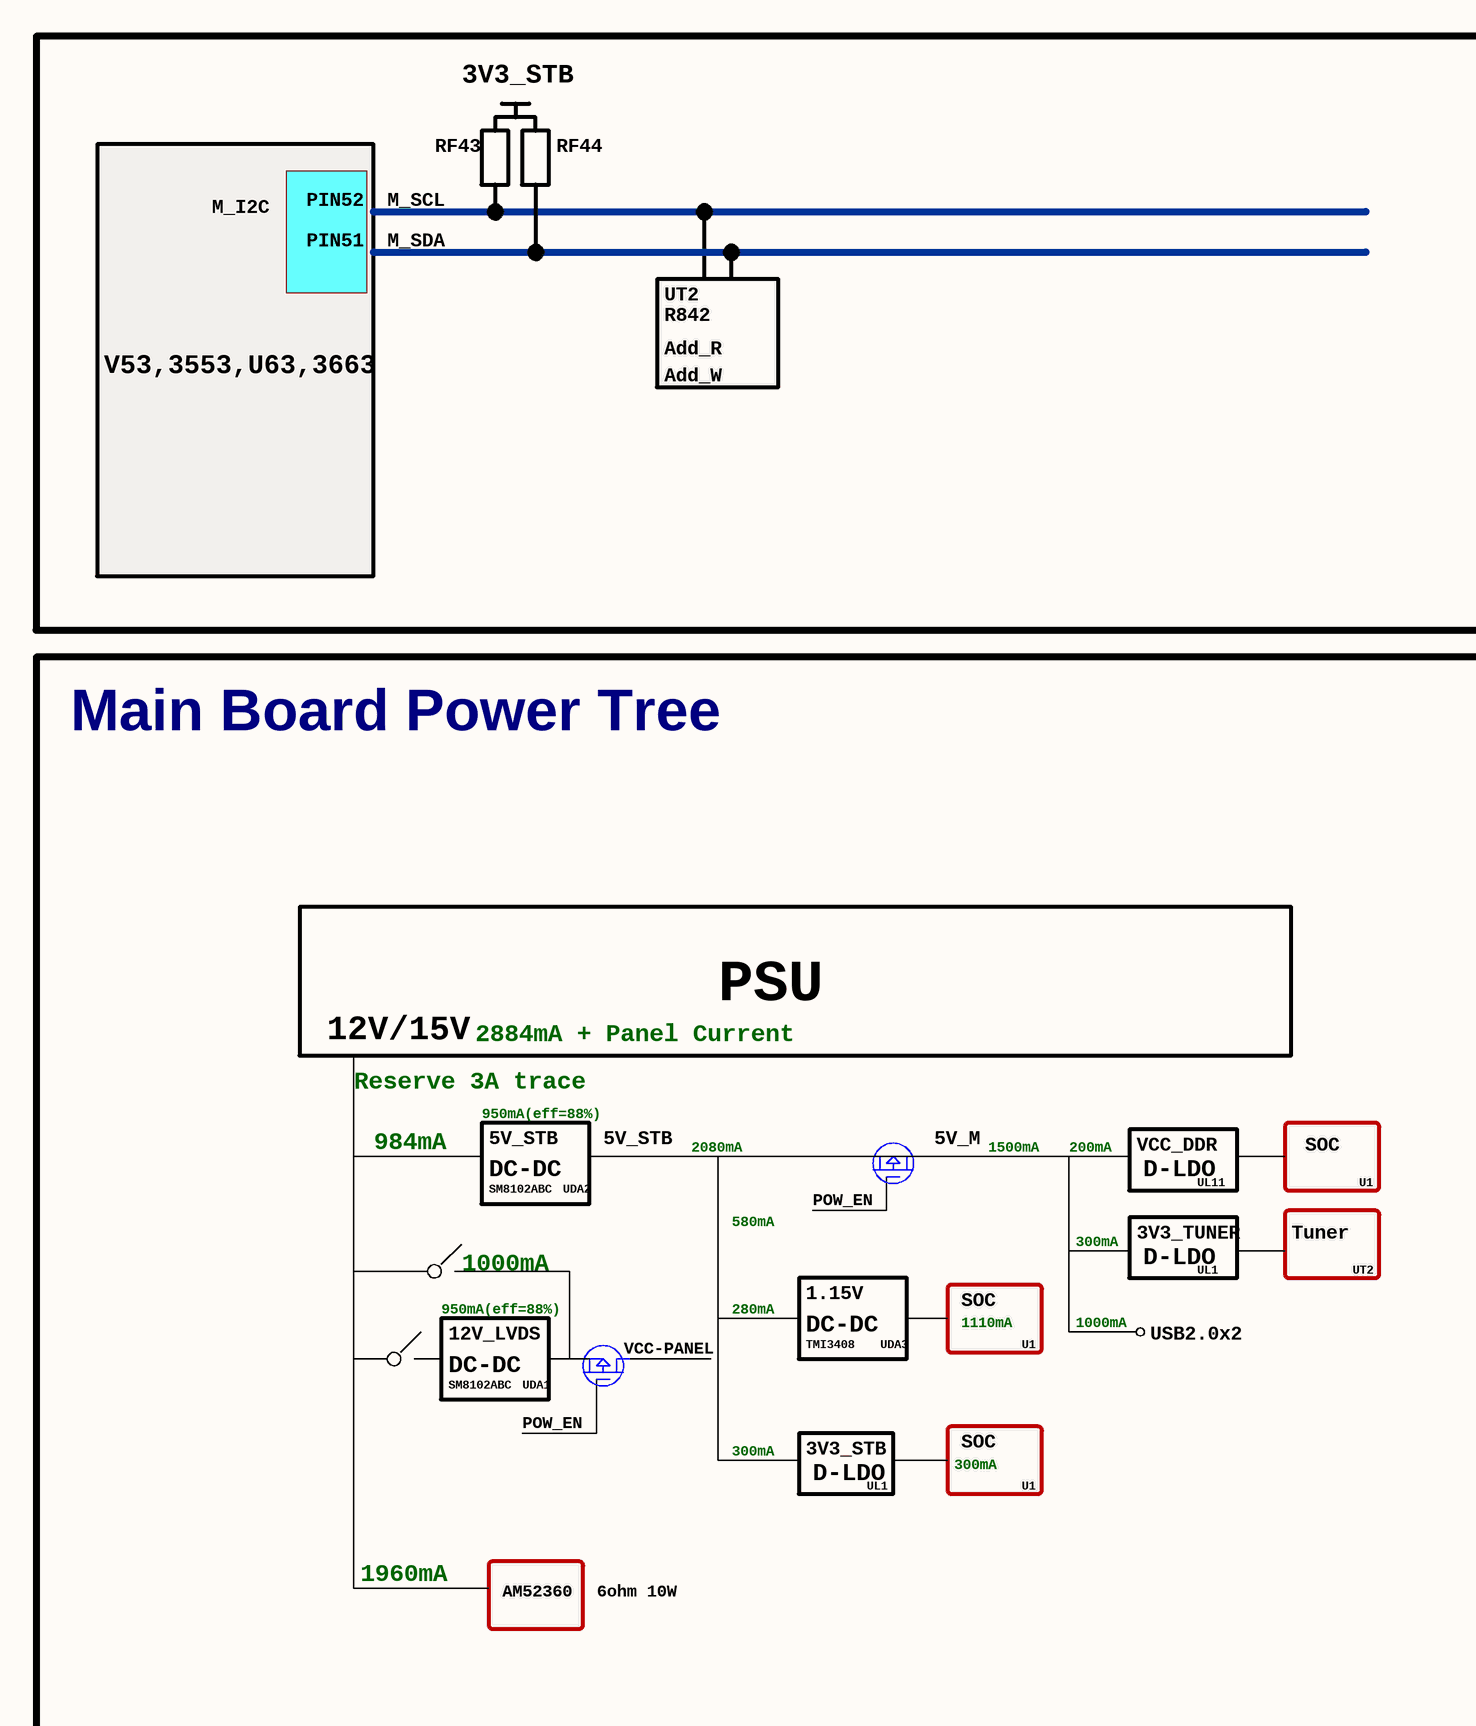
[diagram p0: MISC105950-34.SchDoc, left]
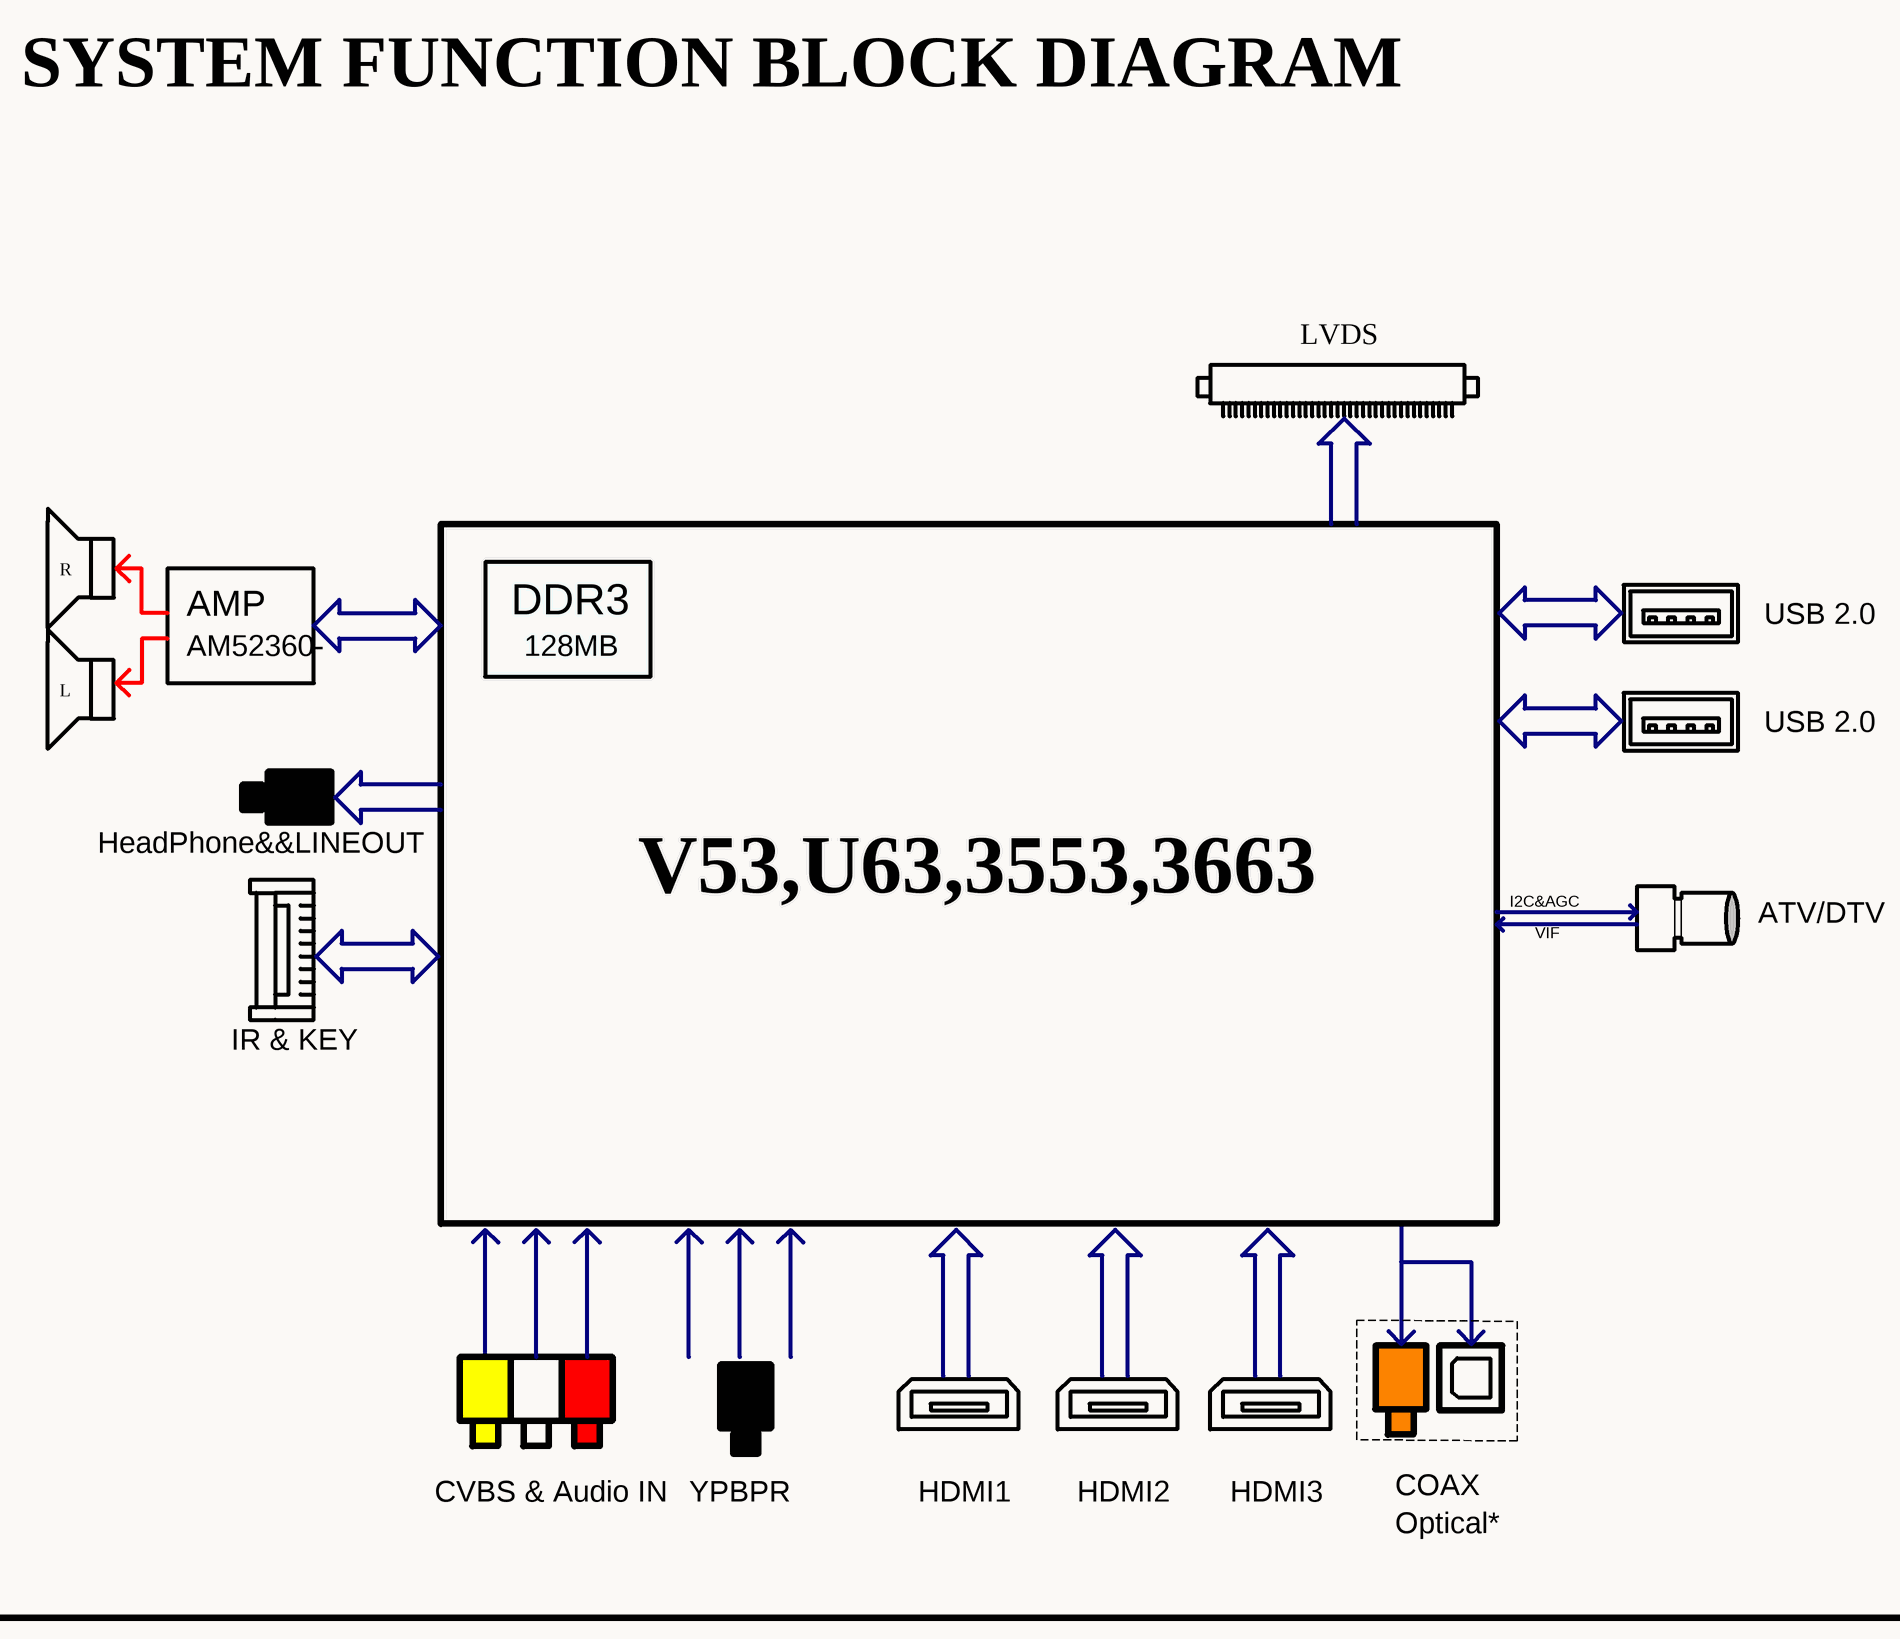
[diagram p1: MISC105950-34.SchDoc, right]
# Altium project MISC105950-48.PrjPCB (part 2 of 8)

## Sheet MISC105950-34.SchDoc
size 762 x 342 mm

### Notes on the sheet
- 3V3_STB
- M_I2C
- PIN52
- M_SCL
- RF43
- RF44
- SYSTEM FUNCTION BLOCK DIAGRAM
- PIN51
- M_SDA
- UT2
- R842
- Add_R
- V53,3553,U63,3663
- Add_W
- LVDS
- R
- Main Board Power Tree
- AMP
- AM52360-
- DDR3
- 128MB
- USB 2.0
- L
- PSU
- HeadPhone&&LINEOUT
- V53,U63,3553,3663
- I2C&AGC
- 12V/15V
- Reserve 3A trace
- 2884mA + Panel Current
- VIF
- ATV/DTV
- 984mA
- 950mA(eff=88%)
- 5V_STB
- 2080mA
- 5V_M
- 1500mA
- 200mA
- VCC_DDR
- SOC
- DC-DC
- SM8102ABC
- UDA2
- 580mA
- POW_EN
- D-LDO
- UL11
- U1
- IR & KEY
- 1000mA
- 1.15V
- 300mA
- 3V3_TUNER
- UL1
- Tuner
- 12V_LVDS
- VCC-PANEL
- 280mA
- TMI3408
- UDA3
- 1110mA
- USB2.0x2
- UDA1
- 1960mA
- AM52360
- 6ohm 10W
- CVBS & Audio IN
- YPBPR
- HDMI1
- HDMI2
- HDMI3
- COAX
- Optical*